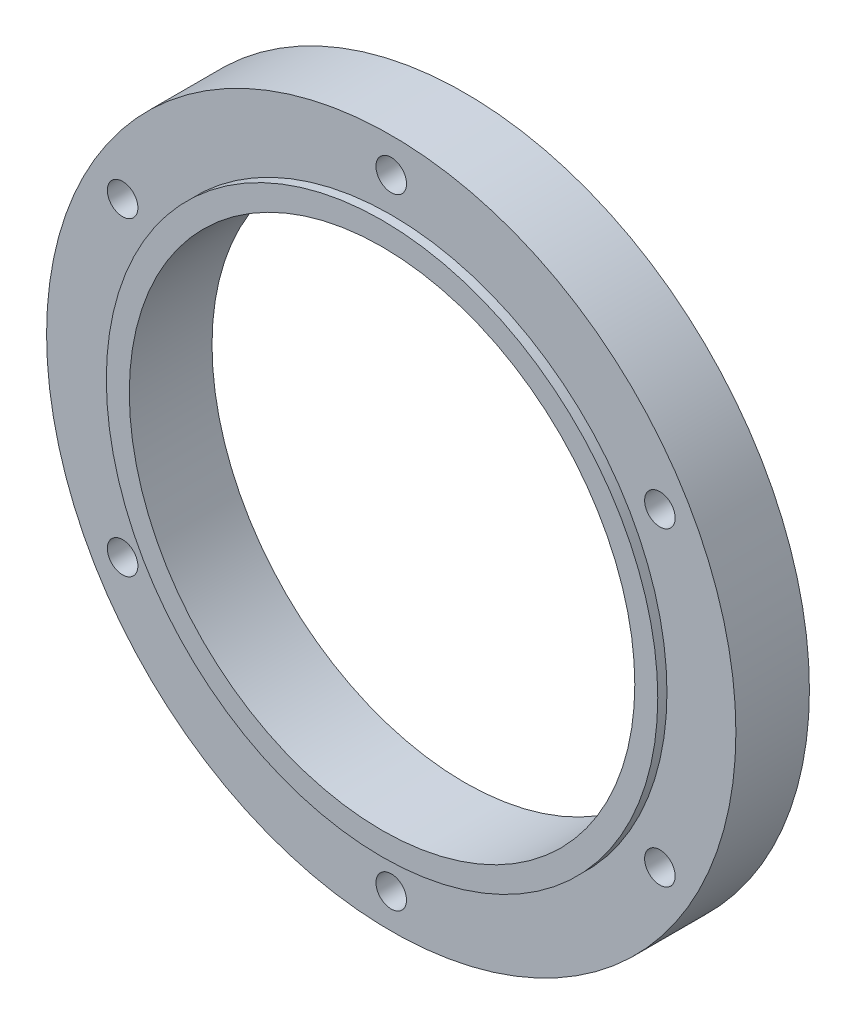
from build123d import *

# Parameters (mm, degrees)
SKETCH1_R           = 75
SKETCH1_R_2         = 55
SKETCH1_R_3         = 3.325
BOSS_EXTRUDE1_DEPTH = 16
SKETCH2_R           = 60
SKETCH2_R_2         = 55
BOSS_EXTRUDE2_DEPTH = 2


with BuildPart() as part:
    # Sketch1 → Boss-Extrude1 (new body)
    with BuildSketch(Plane.XY):
        Circle(SKETCH1_R)
        Circle(SKETCH1_R_2, mode=Mode.SUBTRACT)
        with Locations((0, 67.5)):
            Circle(SKETCH1_R_3, mode=Mode.SUBTRACT)
        with Locations((58.456714755, 33.75)):
            Circle(SKETCH1_R_3, mode=Mode.SUBTRACT)
        with Locations((58.456714755, -33.75)):
            Circle(SKETCH1_R_3, mode=Mode.SUBTRACT)
        with Locations((0, -67.5)):
            Circle(SKETCH1_R_3, mode=Mode.SUBTRACT)
        with Locations((-58.456714755, -33.75)):
            Circle(SKETCH1_R_3, mode=Mode.SUBTRACT)
        with Locations((-58.456714755, 33.75)):
            Circle(SKETCH1_R_3, mode=Mode.SUBTRACT)
    extrude(amount=BOSS_EXTRUDE1_DEPTH)

    # Sketch2 → Boss-Extrude2 (add)
    with BuildSketch(Plane.XY.offset(16)):
        Circle(SKETCH2_R)
        Circle(SKETCH2_R_2, mode=Mode.SUBTRACT)
    extrude(amount=BOSS_EXTRUDE2_DEPTH)


solid = part.part
